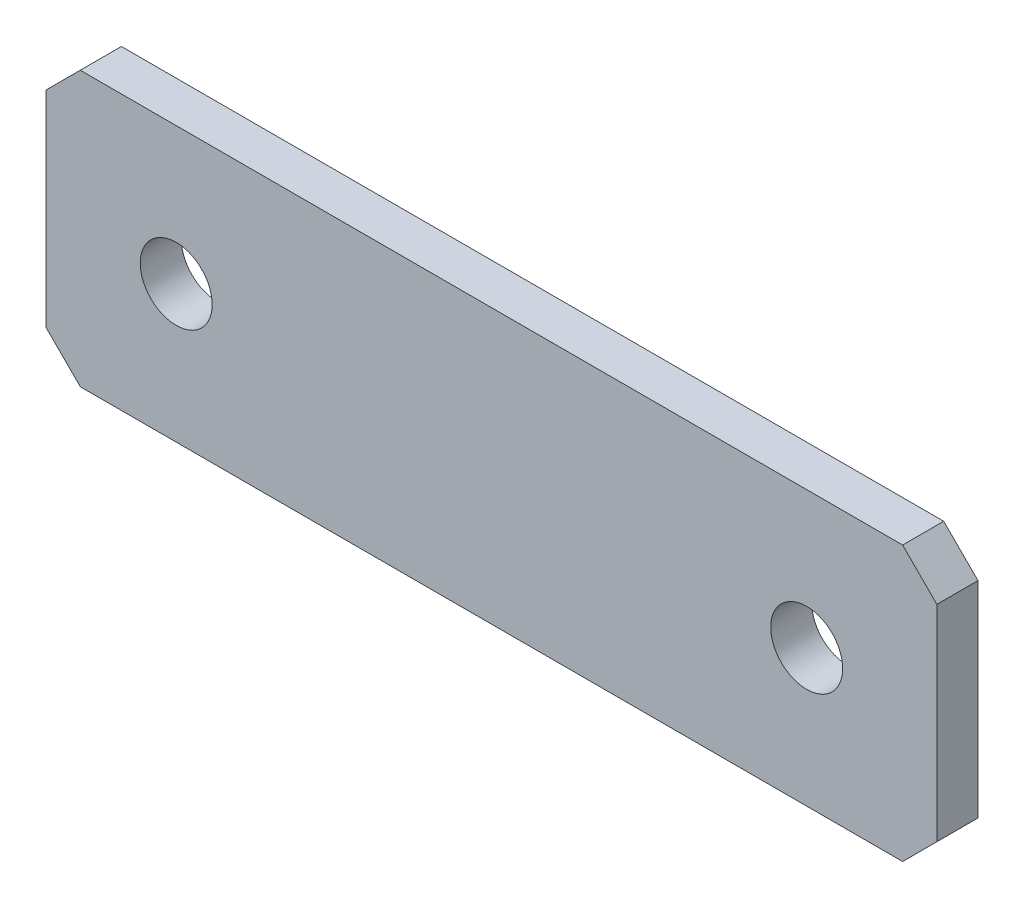
SolidWorks part; units mm, degrees
material "1023 碳钢板 (SS)"
ref_plane "Front Plane" through (0, 0, 0) normal (0, 0, 1) x (1, 0, 0)
ref_plane "Top Plane" through (0, 0, 0) normal (0, 1, 0) x (1, 0, 0)
ref_plane "Right Plane" through (0, 0, 0) normal (1, 0, 0) x (0, 0, -1)
sketch "Sketch1" plane through (0, 0, 0) normal (0, 0, 1) x (1, 0, 0)
  line L0 (-65, 15) -> (-60, 20)
  line L1 (60, -20) -> (-60, -20)
  line L2 (65, -15) -> (65, 15)
  line L3 (60, 20) -> (-60, 20)
  line L4 (-65, -15) -> (-65, 15)
  line L5 (65, -20) -> (-65, 20) construction
  line L6 (65, 20) -> (-65, -20) construction
  line L7 (-60, -20) -> (-65, -15)
  line L8 (65, -15) -> (60, -20)
  line L9 (65, 15) -> (60, 20)
  line L10 (0, 20) -> (0, -20) construction
  line L11 (-65, 0) -> (65, 0) construction
  circle A0 centre (-46, 0) radius 5.25
  circle A1 centre (46, 0) radius 5.25
  point P0 (0, 0)
  dimension "D3" = 10.5
  dimension "D4" = 92
  dimension "D1" = 130
  dimension "D2" = 40
extrude "Boss-Extrude1" add sketch "Sketch1" along normal mid plane 6
